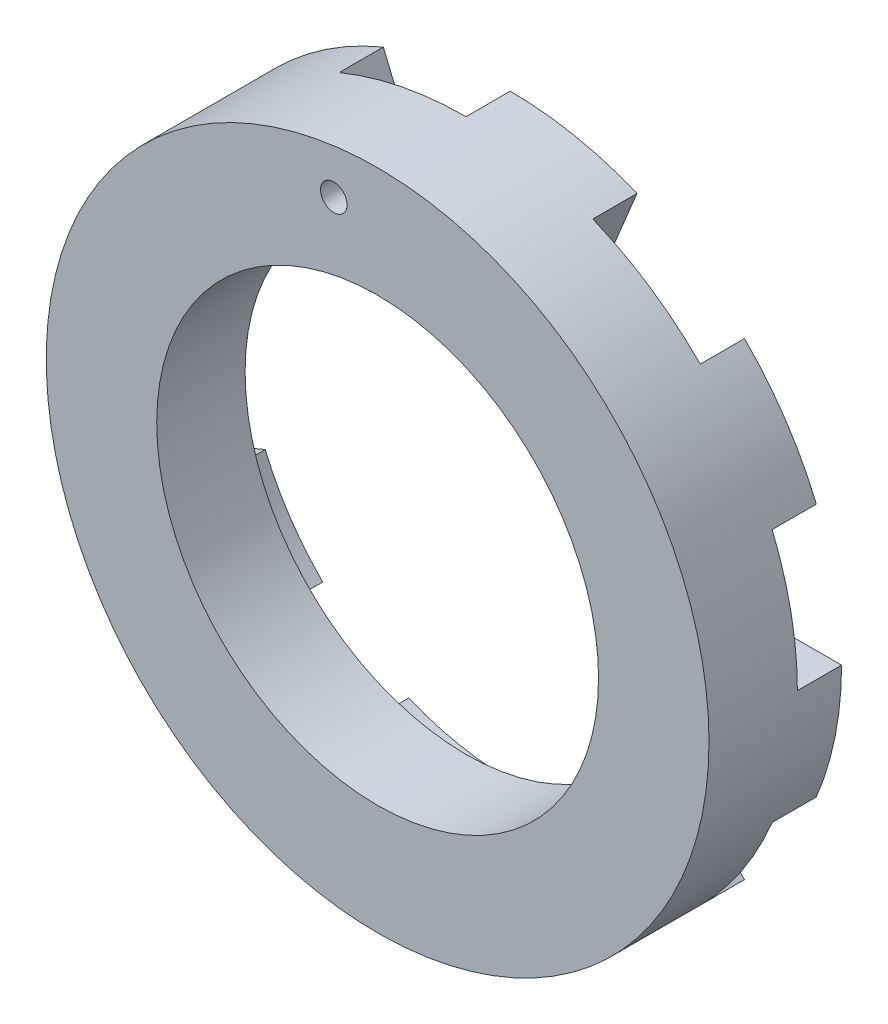
SolidWorks part; units mm, degrees
ref_plane "Front Plane" through (0, 0, 0) normal (0, 0, 1) x (1, 0, 0)
ref_plane "Top Plane" through (0, 0, 0) normal (0, 1, 0) x (1, 0, 0)
ref_plane "Right Plane" through (0, 0, 0) normal (1, 0, 0) x (0, 0, -1)
sketch "Sketch1" plane through (0, 0, 0) normal (0, 0, 1) x (1, 0, 0)
  circle A0 centre (0, 0) radius 25
  circle A1 centre (0, 0) radius 37.5
  dimension "D1" = 50
  dimension "D2" = 75
extrude "Boss-Extrude1" add sketch "Sketch1" along normal blind 15
sketch "Sketch2" plane through (0, 0, 0) normal (0, 0, -1) x (-1, 0, 0)
  circle A0 centre (0, 0) radius 30
  dimension "D1" = 60
extrude "Cut-Extrude1" cut sketch "Sketch2" against normal blind 5
sketch "Sketch3" plane through (0, 0, 0) normal (0, 0, -1) x (-1, 0, 0)
  line L0 (0, 30) -> (0, 37.5)
  line L1 (11.4805, 27.7164) -> (14.3506, 34.6455)
  line L2 (21.2132, 21.2132) -> (26.5165, 26.5165)
  line L3 (27.7164, 11.4805) -> (34.6455, 14.3506)
  line L4 (30, 0) -> (37.5, 0)
  line L5 (27.7164, -11.4805) -> (34.6455, -14.3506)
  line L6 (21.2132, -21.2132) -> (26.5165, -26.5165)
  line L7 (11.4805, -27.7164) -> (14.3506, -34.6455)
  line L8 (0, -30) -> (0, -37.5)
  line L9 (-11.4805, -27.7164) -> (-14.3506, -34.6455)
  line L10 (-21.2132, -21.2132) -> (-26.5165, -26.5165)
  line L11 (-27.7164, -11.4805) -> (-34.6455, -14.3506)
  line L12 (-30, 0) -> (-37.5, 0)
  line L13 (-27.7164, 11.4805) -> (-34.6455, 14.3506)
  line L14 (-21.2132, 21.2132) -> (-26.5165, 26.5165)
  line L15 (-11.4805, 27.7164) -> (-14.3506, 34.6455)
  arc A0 (-14.3506, 34.6455) -> (-26.5165, 26.5165) centre (0, 0) ccw
  arc A1 (-11.4805, 27.7164) -> (-21.2132, 21.2132) centre (0, 0) ccw
  arc A2 (14.3506, 34.6455) -> (0, 37.5) centre (0, 0) ccw
  arc A3 (11.4805, 27.7164) -> (0, 30) centre (0, 0) ccw
  arc A4 (34.6455, 14.3506) -> (26.5165, 26.5165) centre (0, 0) ccw
  arc A5 (27.7164, 11.4805) -> (21.2132, 21.2132) centre (0, 0) ccw
  arc A6 (27.7164, -11.4805) -> (30, 0) centre (0, 0) ccw
  arc A7 (34.6455, -14.3506) -> (37.5, 0) centre (0, 0) ccw
  arc A8 (14.3506, -34.6455) -> (26.5165, -26.5165) centre (0, 0) ccw
  arc A9 (11.4805, -27.7164) -> (21.2132, -21.2132) centre (0, 0) ccw
  arc A10 (-11.4805, -27.7164) -> (0, -30) centre (0, 0) ccw
  arc A11 (-14.3506, -34.6455) -> (0, -37.5) centre (0, 0) ccw
  arc A12 (-34.6455, -14.3506) -> (-26.5165, -26.5165) centre (0, 0) ccw
  arc A13 (-27.7164, -11.4805) -> (-21.2132, -21.2132) centre (0, 0) ccw
  arc A14 (-27.7164, 11.4805) -> (-30, 0) centre (0, 0) ccw
  arc A15 (-34.6455, 14.3506) -> (-37.5, 0) centre (0, 0) ccw
  point P23 (0, 0)
  dimension "D1" = 16
extrude "Cut-Extrude2" cut sketch "Sketch3" against normal blind 5
sketch "Sketch4" plane through (0, 0, 5) normal (0, 0, -1) x (-1, 0, 0)
  circle A0 centre (0, 0) radius 32.5 construction
  circle A1 centre (4.9605, 32.1192) radius 1.5
  dimension "D1" = 65
  dimension "D2" = 3
extrude "Cut-Extrude3" cut sketch "Sketch4" against normal blind 10
